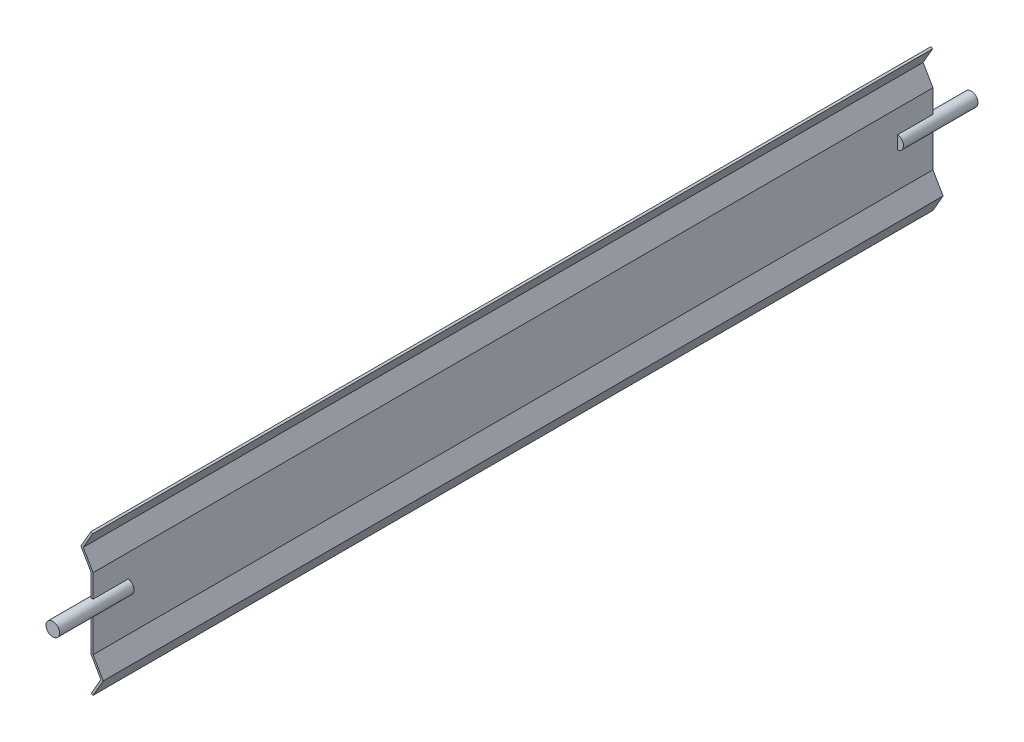
from build123d import *

# Parameters (mm, degrees)
BOSS_EXTRUDE1_DEPTH = 310
BOSS_EXTRUDE2_START = -26
SKETCH2_R           = 5
BOSS_EXTRUDE2_DEPTH = 55


with BuildPart() as part:
    # Sketch1 → Boss-Extrude1 (new, symmetric)
    with BuildSketch(Plane.XY):
        Polygon((0, 0), (7.5, 12.990381057), (0, 25.980762114), (0, 78.421161675), (-7.267949192, 91.009618943), (-0.200961894, 103.25), (-1.5, 104), (-9, 91.009618943), (-1.5, 78.019237886), (-1.5, 25.578838325), (5.767949192, 12.990381057), (-1.299038106, 0.75), align=None)
    extrude(amount=BOSS_EXTRUDE1_DEPTH, both=True)

    # Sketch2 → Boss-Extrude2 (add)
    with BuildSketch(Plane.XY.offset(310).offset(BOSS_EXTRUDE2_START)):
        with Locations((-0.75, 56.5)):
            Circle(SKETCH2_R)
    boss_extrude2 = extrude(amount=BOSS_EXTRUDE2_DEPTH)

    # Mirror1: Boss-Extrude2 across plane
    add(boss_extrude2.mirror(Plane.XY))


solid = part.part
